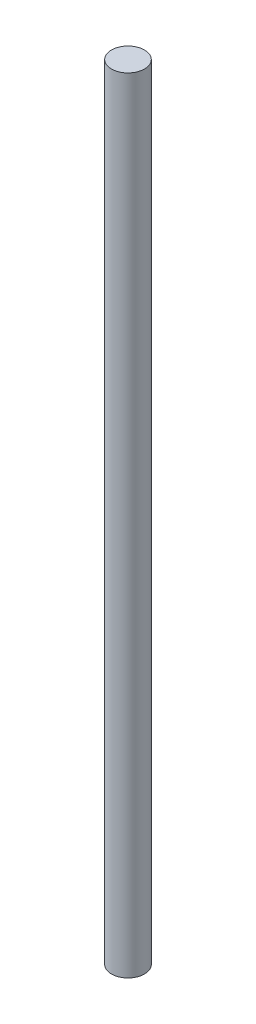
from build123d import *

# Parameters (mm, degrees)
SKETCH1_R           = 8
BOSS_EXTRUDE1_DEPTH = 380


with BuildPart() as part:
    # Sketch1 → Boss-Extrude1 (new body)
    with BuildSketch(Plane(origin=(0, 0, 0), x_dir=(1, 0, 0), z_dir=(0, 1, 0))):
        with Locations(Location((0, 0, 0), (0, 0, 270))):
            Circle(SKETCH1_R)
    extrude(amount=BOSS_EXTRUDE1_DEPTH)


solid = part.part
